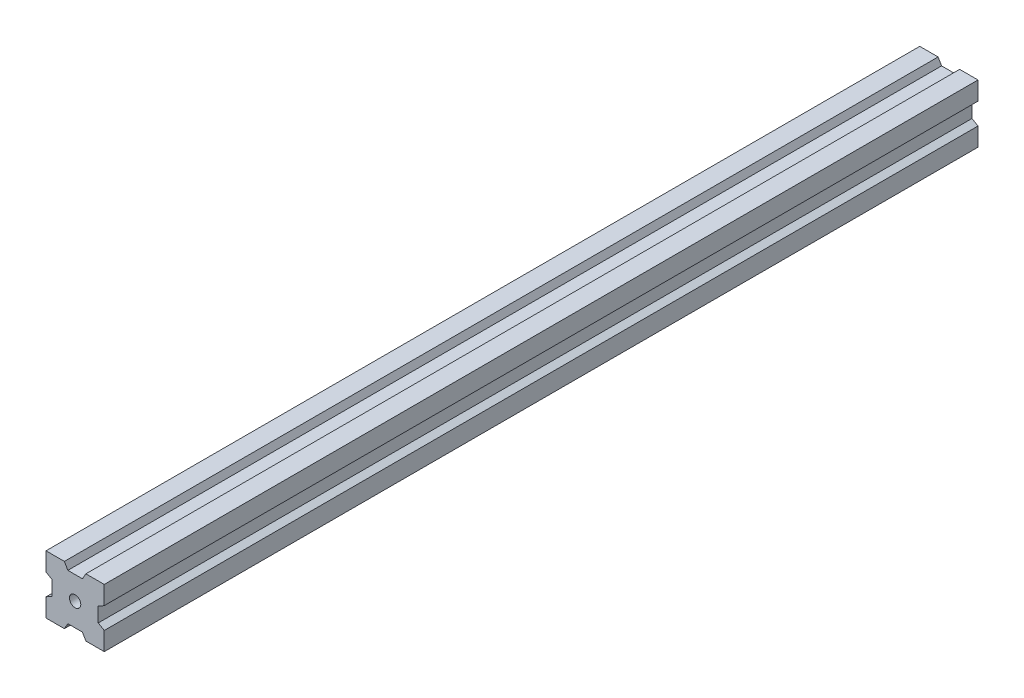
SolidWorks part; units mm, degrees
ref_plane "前视基准面" through (0, 0, 0) normal (0, 0, 1) x (1, 0, 0)
ref_plane "上视基准面" through (0, 0, 0) normal (0, 1, 0) x (1, 0, 0)
ref_plane "右视基准面" through (0, 0, 0) normal (1, 0, 0) x (0, 0, -1)
sketch "草图1" plane through (0, 0, 0) normal (0, 0, 1) x (1, 0, 0)
  line L1 (10, -10) -> (-10, -10)
  line L2 (10, -10) -> (10, 10)
  line L3 (10, 10) -> (-10, 10)
  line L4 (-10, -10) -> (-10, 10)
  line L5 (10, -10) -> (-10, 10) construction
  line L6 (10, 10) -> (-10, -10) construction
  circle A0 centre (0, 0) radius 1.9444
  point P0 (0, 0)
  dimension "D1" = 20
extrude "凸台-拉伸1" add sketch "草图1" along normal mid plane 300
sketch "草图2" plane through (0, 0, 150) normal (0, 0, 1) x (1, 0, 0)
  line L0 (-3.6944, 10) -> (-2.5, 7.9312)
  line L1 (10, 10) -> (-10, 10) construction
  line L2 (-2.5, 7.9312) -> (2.5, 7.9312)
  line L3 (2.5, 7.9312) -> (3.6944, 10)
  line L4 (0, 10) -> (0, 7.9312) construction
  line L5 (-3.6944, 10) -> (3.6944, 10) construction
  dimension "D1" = 5
  dimension "D2" = 60
extrude "切除-拉伸1" cut sketch "草图2" against normal through all and the other way through all
pattern_circular "阵列(圆周)1" count 4 over 360 about axis through (0, 0, 150) along (0, 0, -1) of "切除-拉伸1"
